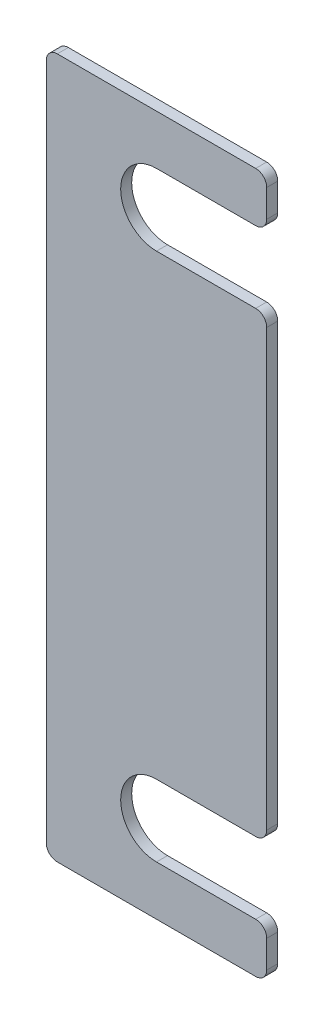
from build123d import *

# Parameters (mm, degrees)
SKETCH_1_W          = 40
SKETCH_1_H          = 127
EXTRUDE_1_DEPTH     = 2
SKETCH_2_R          = 6.5
CUT_EXTRUDE_1_DEPTH = 3
SKETCH_4_W          = 20
SKETCH_4_H          = 13
CUT_EXTRUDE_4_DEPTH = 10
FILLET_2_R          = 2


with BuildPart() as part:
    # 草图1 → 凸台-拉伸1 (new body)
    with BuildSketch(Plane.XY):
        Rectangle(SKETCH_1_W, SKETCH_1_H)
    extrude(amount=EXTRUDE_1_DEPTH)

    # 草图2 → 切除-拉伸1 (cut)
    with BuildSketch(Plane.XY.offset(2)):
        with Locations((0, 48)):
            Circle(SKETCH_2_R)
        with Locations((0, -48)):
            Circle(SKETCH_2_R)
    extrude(amount=-CUT_EXTRUDE_1_DEPTH, mode=Mode.SUBTRACT)

    # 草图4 → 切除-拉伸4 (cut)
    with BuildSketch(Plane.XY.offset(2)):
        with Locations((10, 48)):
            Rectangle(SKETCH_4_W, SKETCH_4_H)
        with Locations((10, -48)):
            Rectangle(SKETCH_4_W, SKETCH_4_H)
    extrude(amount=-CUT_EXTRUDE_4_DEPTH, mode=Mode.SUBTRACT)

    # 圆角2
    fillet_2_edges = [part.edges().sort_by_distance(p)[0] for p in [
        (20, 54.5, 1),
        (20, 41.5, 1),
        (20, -41.5, 1),
        (20, -54.5, 1),
        (-20, 63.5, 1),
        (20, 63.5, 1),
        (20, -63.5, 1),
        (-20, -63.5, 1),
    ]]
    fillet(fillet_2_edges, radius=FILLET_2_R)


solid = part.part
